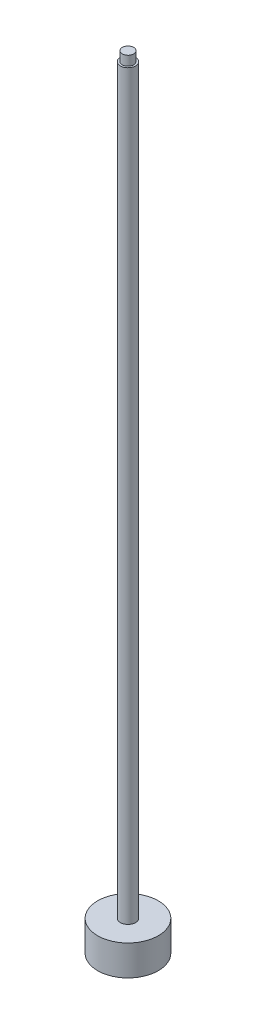
SolidWorks part; units mm, degrees
material "Q235B"
ref_plane "Front Plane" through (0, 0, 0) normal (0, 0, 1) x (1, 0, 0)
ref_plane "Top Plane" through (0, 0, 0) normal (0, 1, 0) x (1, 0, 0)
ref_plane "Right Plane" through (0, 0, 0) normal (1, 0, 0) x (0, 0, -1)
sketch "Sketch1" plane through (0, 0, 0) normal (0, 0, 1) x (1, 0, 0)
  line L0 (0, 0) -> (30, 0)
  line L1 (30, 0) -> (30, 50)
  line L2 (30, 50) -> (160, 50)
  line L3 (160, 50) -> (160, 210)
  line L4 (160, 210) -> (40, 210)
  line L5 (40, 210) -> (40, 4126)
  line L6 (40, 4126) -> (30, 4126)
  line L7 (30, 4126) -> (30, 4176)
  line L8 (30, 4176) -> (0, 4176)
  line L9 (0, 4176) -> (0, 0) construction
  line L10 (0, 0) -> (0, 4176)
  dimension "D1" = 80
  dimension "D2" = 60
  dimension "D3" = 60
  dimension "D4" = 160
  dimension "D5" = 50
  dimension "D6" = 3966
  dimension "D7" = 50
  dimension "D8" = 320
revolve "Revolve1" add sketch "Sketch1" angle 360 about L9
